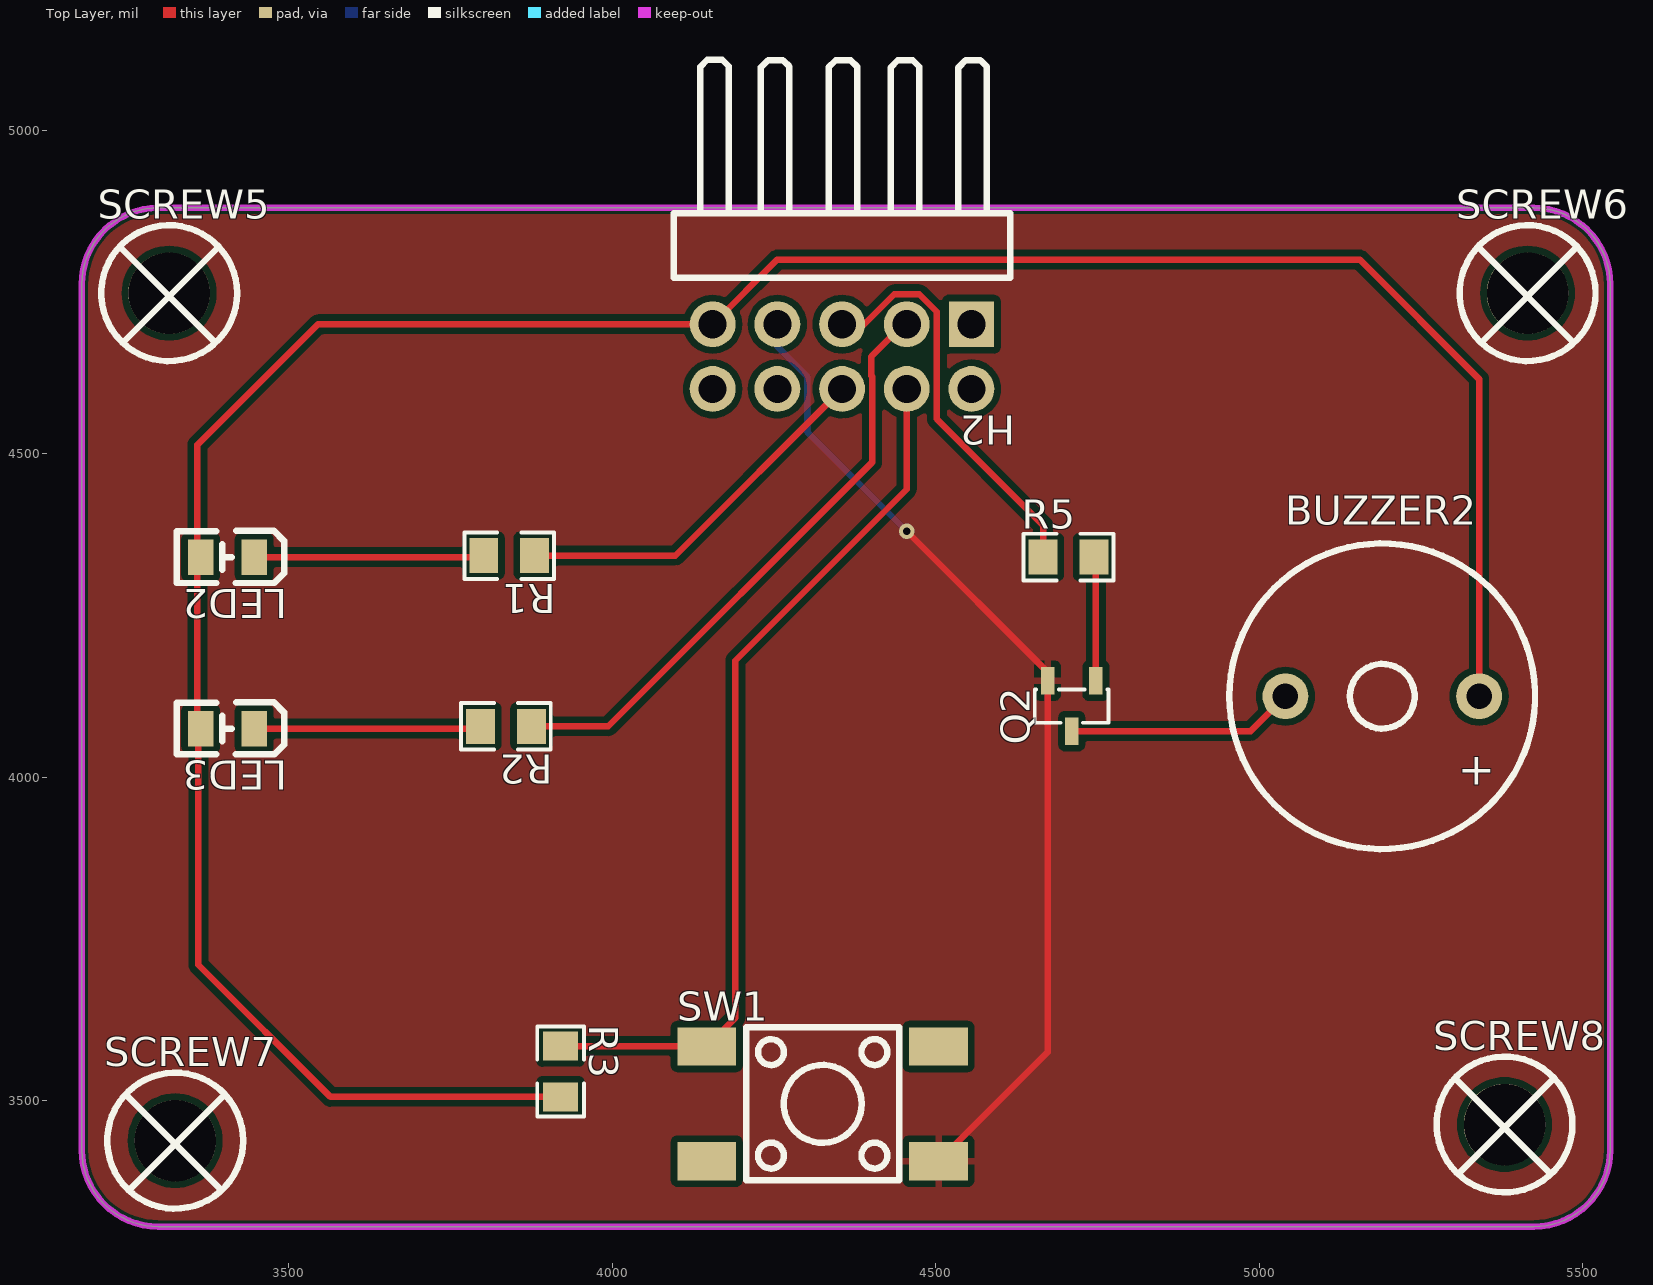
[diagram p0: Top Layer view]
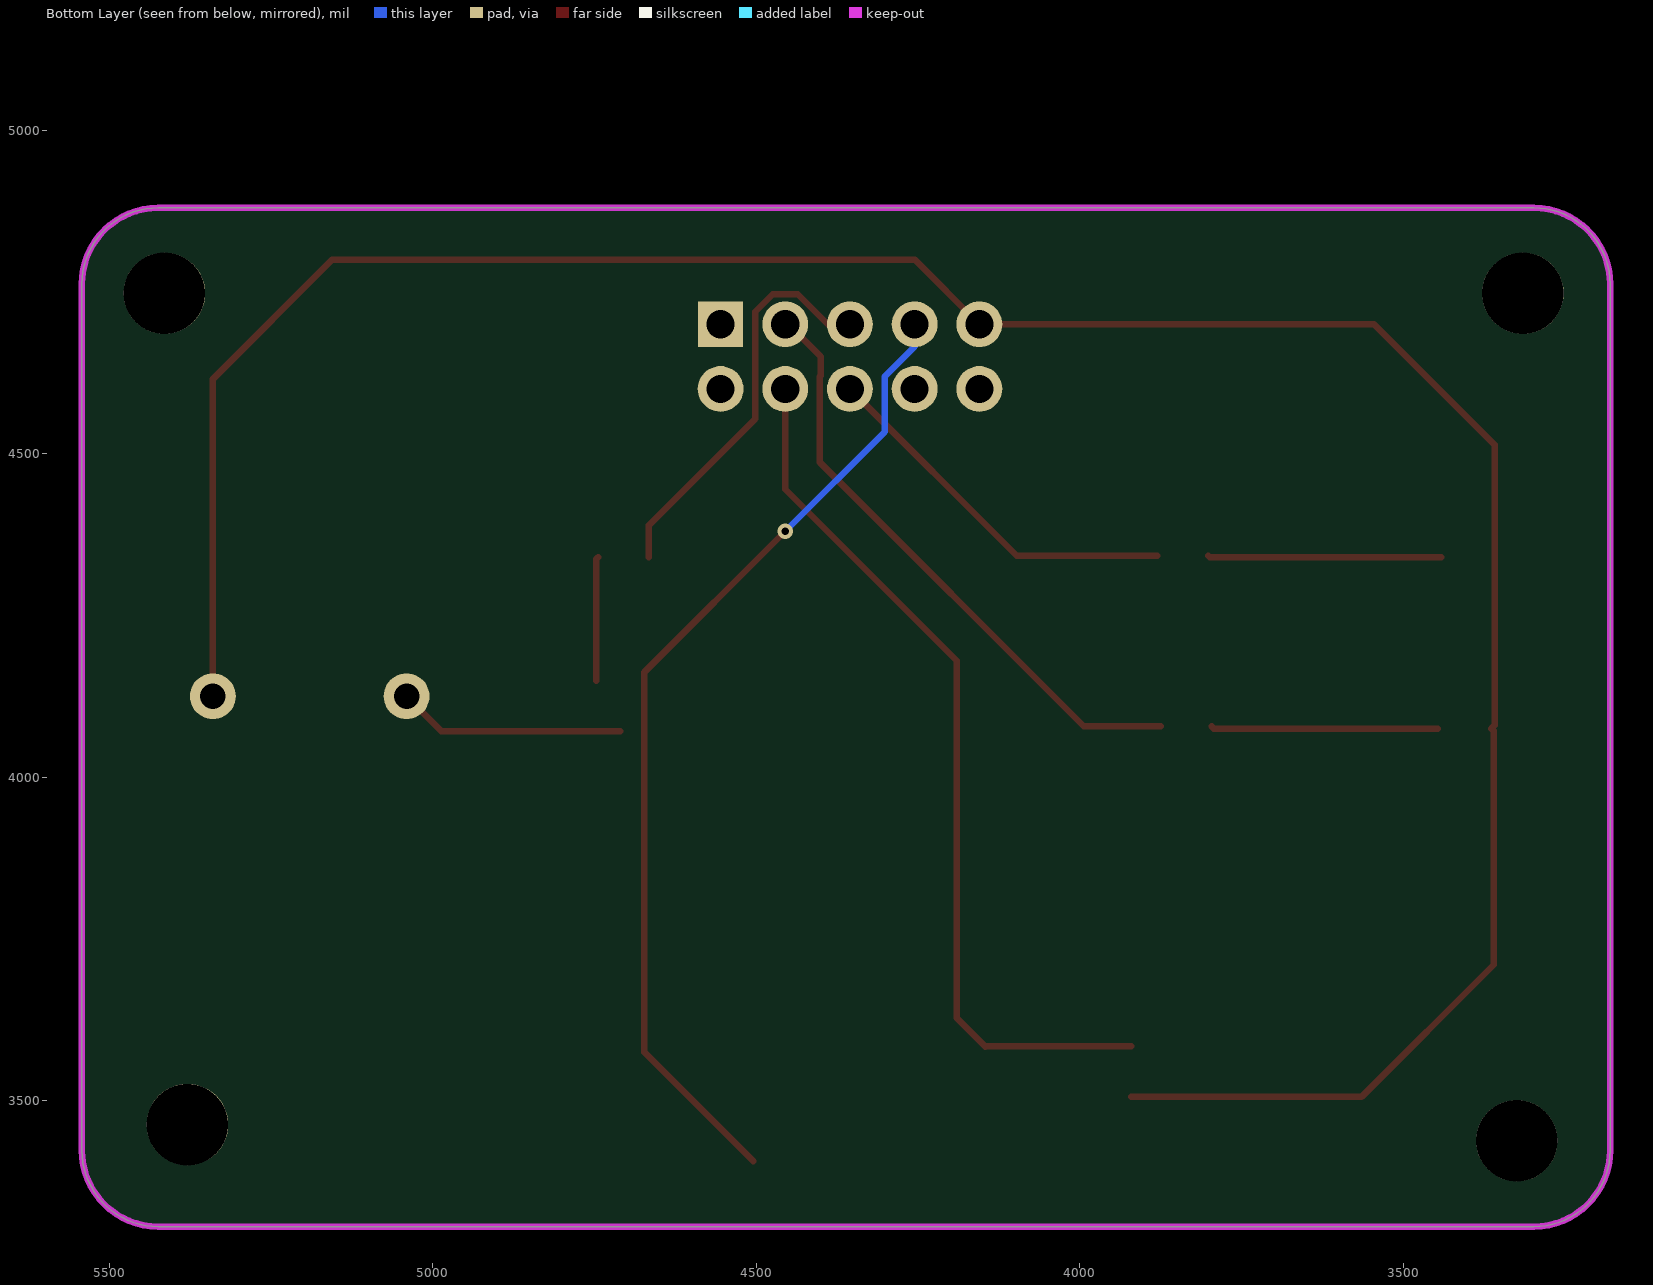
[diagram p1: Bottom Layer view, seen from below]
# Altium PCB MISC89027.pcbdoc
Units mil, origin at the board's own origin, x right, y up, seen from the top; angles counter-clockwise.
Board outline 2362.2 x 1574.8 mil, 2 copper layers (Top Layer, Bottom Layer), stack 62.206 mil thick; 14 components, 16 nets, 35 pads, 1 vias.

## Layer stack, top to bottom
Top Solder Mask Layer: solder mask 0.394, Dk 3.3
Top Layer: signal copper 1.379
Dielectric1: surface 59.449, FR4, Dk 4.5
Bottom Layer: signal copper 1.378
Bottom Solder Mask Layer: solder mask 0.394, Dk 3.3

## Board outline
3298.11,4880 ccw(c3298.11,4761.89) 3180,4761.89 3180,3423.31 ccw(c3298.11,3423.31) 3298.11,3305.2 5424.09,3305.2 ccw(c5424.09,3423.31) 5542.2,3423.31 5542.2,4761.89 ccw(c5424.09,4761.89) 5424.09,4880

## Design rules (kind name [scope] priority, off if disabled: settings)
BoardOutlineClearance copperThickness2oz_1 [All] p2 off: genericclearance=7.99 ignorepadtopadclearanceinfootprint=FALSE except(0: Arc-SplitContinuation Track-SplitContinuation SMDPad-SplitContinuation THPad-SplitContinuation Via-SplitContinuation Fill-SplitContinuation Region-SplitContinuation Poly-SplitContinuation Text-SplitContinuation Hole-SplitContinuation; 5.98: Arc-CutoutEdge SMDPad-CutoutEdge THPad-CutoutEdge Via-CutoutEdge Fill-CutoutEdge Region-CutoutEdge Text-CutoutEdge; 6.93: Hole-OutlineEdge Hole-CutoutEdge; 10: Poly-OutlineEdge Poly-CutoutEdge; 11.81: Arc-OutlineEdge Track-OutlineEdge SMDPad-OutlineEdge THPad-OutlineEdge Via-OutlineEdge Fill-OutlineEdge Region-OutlineEdge Text-OutlineEdge Track-CutoutEdge)
BoardOutlineClearance copperThickness1oz_1 [All] p4: genericclearance=4.02 ignorepadtopadclearanceinfootprint=FALSE except(0: Arc-SplitContinuation Track-SplitContinuation SMDPad-SplitContinuation THPad-SplitContinuation Via-SplitContinuation Fill-SplitContinuation Region-SplitContinuation Poly-SplitContinuation Text-SplitContinuation Hole-SplitContinuation; 6: SMDPad-CutoutEdge THPad-CutoutEdge Via-CutoutEdge Fill-CutoutEdge Region-CutoutEdge Text-CutoutEdge; 6.93: Hole-OutlineEdge Hole-CutoutEdge; 10: Poly-OutlineEdge Poly-CutoutEdge; 11.8: Arc-OutlineEdge Track-OutlineEdge SMDPad-OutlineEdge THPad-OutlineEdge Via-OutlineEdge Fill-OutlineEdge Region-OutlineEdge Text-OutlineEdge; 11.81: Arc-CutoutEdge Track-CutoutEdge)
Clearance copperThickness2oz [All] p1 off: gap=7.99 ignorepadtopadclearanceinfootprint=FALSE except(5.98: SMDPad-Track SMDPad-SMDPad THPad-Track SMDPad-THPad THPad-THPad Track-Via SMDPad-Via THPad-Via Via-Via Fill-Track Region-Track Fill-SMDPad Region-SMDPad Fill-THPad Region-THPad Fill-Via Region-Via Fill-Fill Fill-Region Region-Region Arc-Track Arc-SMDPad Arc-THPad Arc-Via Fill-Arc Region-Arc Arc-Arc Text-Track SMDPad-Text Text-THPad Text-Via Fill-Text Region-Text Arc-Text Text-Text; 6.93: Hole-Track Hole-SMDPad Hole-THPad Hole-Via Fill-Hole Region-Hole Hole-Arc Hole-Text; 10: Poly-Track Poly-SMDPad Poly-THPad Poly-Via Poly-Fill Poly-Region Poly-Poly Poly-Arc Poly-Text Poly-Hole)
Clearance copperThickness1oz [All] p3: gap=4.02 ignorepadtopadclearanceinfootprint=FALSE except(0: THPad-Track Hole-Track; 5.98: SMDPad-Track SMDPad-SMDPad SMDPad-THPad THPad-THPad Track-Via SMDPad-Via THPad-Via Via-Via Fill-Track Region-Track Fill-SMDPad Region-SMDPad Fill-THPad Region-THPad Fill-Via Region-Via Fill-Fill Fill-Region Region-Region; 6: Arc-Track Arc-SMDPad Arc-THPad Arc-Via Fill-Arc Region-Arc Arc-Arc Text-Track SMDPad-Text Text-THPad Text-Via Fill-Text Region-Text Arc-Text Text-Text; 6.93: Hole-SMDPad Hole-THPad Hole-Via Fill-Hole Region-Hole Hole-Arc Hole-Text; 10: Poly-Track Poly-SMDPad Poly-THPad Poly-Via Poly-Fill Poly-Region Poly-Poly Poly-Arc Poly-Text Poly-Hole)
DiffPairsRouting differentialPair [All] p1: maxlimit=6 minlimit=6 mostfreqgap=6 toplayer_minwidth=5 toplayer_prefwidth=10 toplayer_maxwidth=100 toplayer_mingap=6 toplayer_prefgap=6 toplayer_maxgap=6 bottomlayer_minwidth=5 bottomlayer_prefwidth=10 bottomlayer_maxwidth=100 bottomlayer_mingap=6 bottomlayer_prefgap=6 bottomlayer_maxgap=6 maxuncoupledlength=10
HoleToHoleClearance otherClearance [All] p1: gap=11.81 allowstackedmicrovias=TRUE
Length netLength [All] p1: minlimit=0 maxlimit=0
MatchedLengths netLengthTolerance [All] p1: tolerance=1000
PasteMaskExpansion pasteMaskExpansion [All] p1: expansion=0
PlaneConnect innerPlane [All] p1: planeconnectstyle=Relief reliefexpansion=20 reliefentries=4 reliefconductorwidth=10 reliefairgap=10
PolygonConnect "copperRegion_Top Layer" [(OnLayer('Top Layer'))] p1: connectstyle=Relief reliefconductorwidth=10 reliefentries=4 polygonreliefangle="90 Angle" airgapwidth=10 via.connectstyle=Relief via.reliefconductorwidth=10 via.reliefentries=4 via.polygonreliefangle="90 Angle" via.airgapwidth=10
PolygonConnect "copperRegion_Bottom Layer" [(OnLayer('Bottom Layer'))] p2: connectstyle=Relief reliefconductorwidth=10 reliefentries=4 polygonreliefangle="90 Angle" airgapwidth=10 via.connectstyle=Relief via.reliefconductorwidth=10 via.reliefentries=4 via.polygonreliefangle="90 Angle" via.airgapwidth=10
PolygonConnect copperRegion [All] p3: connectstyle=Direct reliefconductorwidth=10 reliefentries=4 polygonreliefangle="90 Angle" airgapwidth=10 via.connectstyle=Relief via.reliefconductorwidth=10 via.reliefentries=4 via.polygonreliefangle="90 Angle" via.airgapwidth=10
RoutingVias viaSize [All] p1: holewidth=12.01 width=24.02 viastyle="Through Hole" minholewidth=11.81 minwidth=19.68 maxholewidth=248.03 maxwidth=393.7
SolderMaskExpansion solderMaskExpansion [IsVia] p1: expansion=-1000 istentingtop=TRUE
SolderMaskExpansion solderMaskExpansion [All] p2: expansion=2 istentingtop=FALSE
Width copperThickness2oz_2 [All] p1 off: maxlimit=100 minlimit=8 preferedwidth=10
Width copperThickness1oz_2 [All] p2: maxlimit=100 minlimit=5 preferedwidth=10

## Components (designator, comment, footprint, x,y, rotation, side; value= is the part's Value field where it differs from the comment)
BUZZER2 "2.4kHZ" BUZ-TH_BD12.0-P7.60-D0.6-FD 5190,4125 r180 top
H2 "PZ254R-12-10P" HDR-TH_10P-P2.54-H-M-R2-C5-S2.54 4355,4650 r180 top
LED2 "GL0805UR01" LED0805-R-RD_RED 3405,4340 r180 top
LED3 "GL0805UR01" LED0805-R-RD_RED 3405,4075 r180 top
Q2 "S8050" SOT-23-3_L2.9-W1.3-P1.90-LS2.3-BR 4710,4110 r90 top
R1 "1k" R0805 3840.48,4342.27 r180 top
R2 "1k" R0805 3835.48,4078.53 r180 top
R3 "4.7k" R0805 3920,3545 r270 top
R5 "1k" R0805 4705,4340 r0 top
SCREW5 "" M3螺丝 3317.4,4745.55 r0 top
SCREW6 "" M3螺丝 5417.09,4745.55 r0 top
SCREW7 "" M3螺丝 3326.77,3435.55 r0 top
SCREW8 "" M3螺丝 5381.45,3460.55 r0 top
SW1 "KH-6X6X5H-STM" SW-SMD_4P-L6.0-W6.0-P4.50-LS9.0_H5.0 4325,3495 r0 top

## Footprints (in the part's own frame and the unit in brackets; to place one, negate y for a bottom-side part, rotate by r counter-clockwise, add the part's x,y. Pads: shape width x height; smd on the part's side, far side on the other; paste and mask are expansions set on the pad)
BUZ-TH_BD12.0-P7.60-D0.6-FD [mil]
  round 70.9 hole 39.4 paste+0 mask+2: 1(-149.6,0) 2(149.6,0)
  silkscreen extent -236,-236 236,236
HDR-TH_10P-P2.54-H-M-R2-C5-S2.54 [mm]
  rect 1.778x1.8 hole 1.1: 1(-5.08,-1.27)
  round 1.8 hole 1.1: 2(-5.08,1.27) 3(-2.54,-1.27) 4(-2.54,1.27) 5(0,-1.27) 6(0,1.27) 7(2.54,-1.27) 8(2.54,1.27) 9(5.08,-1.27) 10(5.08,1.27)
  silkscreen extent -6.6,-11.65 6.6,-3.09
LED0805-R-RD_RED [mm]
  rect 1x1.4 smd: 1(1.05,0) 2(-1.05,0)
  silkscreen extent -2.22,-1.04 1.99,1.01
M3螺丝 [mil]
  round 126 hole 126 paste+0 mask+4: 1(-2.5,2.5)
  silkscreen extent -107,-102 102,107
R0805 [mm]
  rect 1.133x1.377 smd paste-100 mask+0.051: 1(-1,0) 2(1,0)
  silkscreen extent -1.76,-0.92 1.76,0.92
SOT-23-3_L2.9-W1.3-P1.90-LS2.3-BR [mm]
  rect 1.07x0.532 smd: 1(0.99,-0.95) 2(0.99,0.95) 3(-0.99,0)
  silkscreen extent -0.66,-1.45 0.64,1.45
SW-SMD_4P-L6.0-W6.0-P4.50-LS9.0_H5.0 [mm]
  rect 2.3x1.5 smd: 1(-4.55,2.25) 2(4.55,2.25) 3(-4.55,-2.25) 4(4.55,-2.25)
  silkscreen extent -3,-3 3,3

## Via types
v1: diameter 24.02, hole 12, Top Layer to Bottom Layer, 1 vias

## Nets (pads, with @x,y where several pads share a name; then routed paths per layer and width w, separated by ;. In a path a pad name is that pad's centre, name@x,y a point inside that pad or via, vN(x,y) a via of type N, cw(c..) or ccw(c..) an arc to the next point about the centre after c; other vN are vias at no path point)
$1N9: R3.1 SW1.1 | length 1370.7
  Top Layer w10: R3.1 4145.09,3584.37 SW1.1 4190,3627.72 4190,4180 4455,4445 4455,4600
$1N23: H2.4
$1N24: H2.6
$1N25: H2.3
$1N26: H2.5
$1N27: H2.7
$1N28: H2.9
$1N30: BUZZER2.2 Q2.3 | length 352.8
  Top Layer w10: Q2.3 4986.41,4071.01 BUZZER2.2
$1N31: Q2.1 R5.2 | length 192.3
  Top Layer w10: R5.2 4747.4,4336.97 Q2.1
$1N32: R5.1 | length 624.2
  Top Layer w10: 4355,4700 4389.36,4700 4435.77,4746.42 4474.23,4746.42 4501.42,4719.23 4501.42,4553.58 4665.63,4389.37 R5.1
$1N34: LED2.2 R1.2 | length 360.7
  Top Layer w10: LED2.2@3441.35,4340 3798.85,4340 R1.2
$1N35: LED3.2 R2.2 | length 351.2
  Top Layer w10: LED3.2 3792.59,4075 R2.2
$1N36: R1.1 | length 581.9
  Top Layer w10: R1.1 4097.27,4342.27 4355,4600
$1N37: R2.1 | length 935.4
  Top Layer w10: R2.1 3993.53,4078.53 4401.42,4486.42 4401.42,4619.23 4400,4620.64 4400,4650 4450,4700 4455,4700
+5V: BUZZER2.1 LED2.1 LED3.1 R3.2 | length 4118.3
  Top Layer w10: R3.2 3564.37,3505.63 3360,3710 3360,4071.35 LED3.1 3358.65,4080 3358.65,4513.65 3545,4700 4155,4700 4255,4800 5155,4800 5339.6,4615.4 BUZZER2.1
GND: Q2.2 SW1.4 | length 1536.3
  Top Layer w10: v1(4455,4380) 4672.6,4162.4 Q2.2 4672.6,3574.89 SW1.4
  Bottom Layer w10: 4255,4700 4255,4665.64 4301.42,4619.23 4301.42,4533.58 v1(4455,4380)
pads on no net: H2.1 H2.2 H2.8 H2.10 SCREW5.1 SCREW6.1 SCREW7.1 SCREW8.1 SW1.2 SW1.3

## Polygon pours and split planes (outlines as drawn)
GND on Top Layer (solid, remove dead copper, pour order 0): 3000,5215 3000,3000 6200,3000 6200,5215

## Keep-outs
Board Outline Layer:
  the board outline again, w10